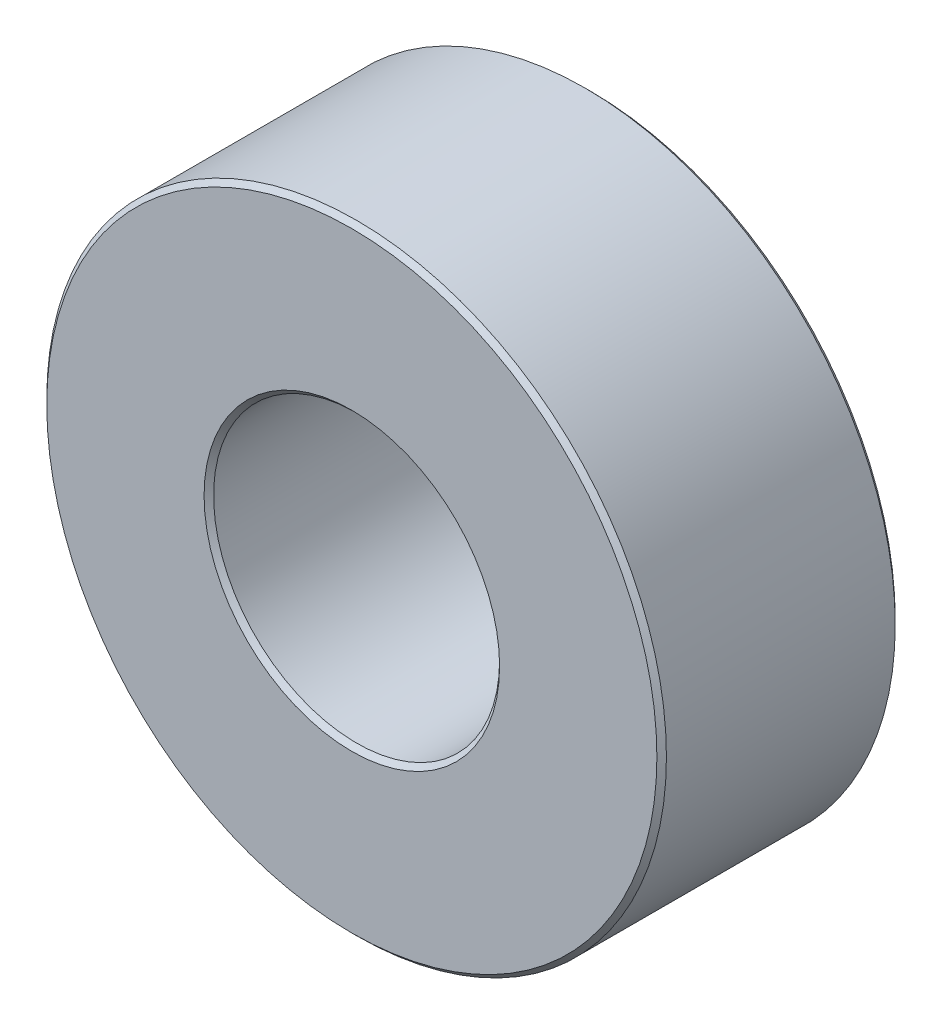
SolidWorks part; units mm, degrees
ref_plane "Front Plane" through (0, 0, 0) normal (0, 0, 1) x (1, 0, 0)
ref_plane "Top Plane" through (0, 0, 0) normal (0, 1, 0) x (1, 0, 0)
ref_plane "Right Plane" through (0, 0, 0) normal (1, 0, 0) x (0, 0, -1)
sketch "Sketch1" plane through (0, 0, 0) normal (0, 0, 1) x (1, 0, 0)
  circle A0 centre (0, 0) radius 6.5
  circle A1 centre (0, 0) radius 3
  dimension "D1" = 13
  dimension "D2" = 6
extrude "Boss-Extrude1" add sketch "Sketch1" along normal blind 5
chamfer "Chamfer1" distance 0.1 angle 45 4 edges at (3, 0, 5) (6.5, 0, 5) (3, 0, 0) (6.5, 0, 0)
